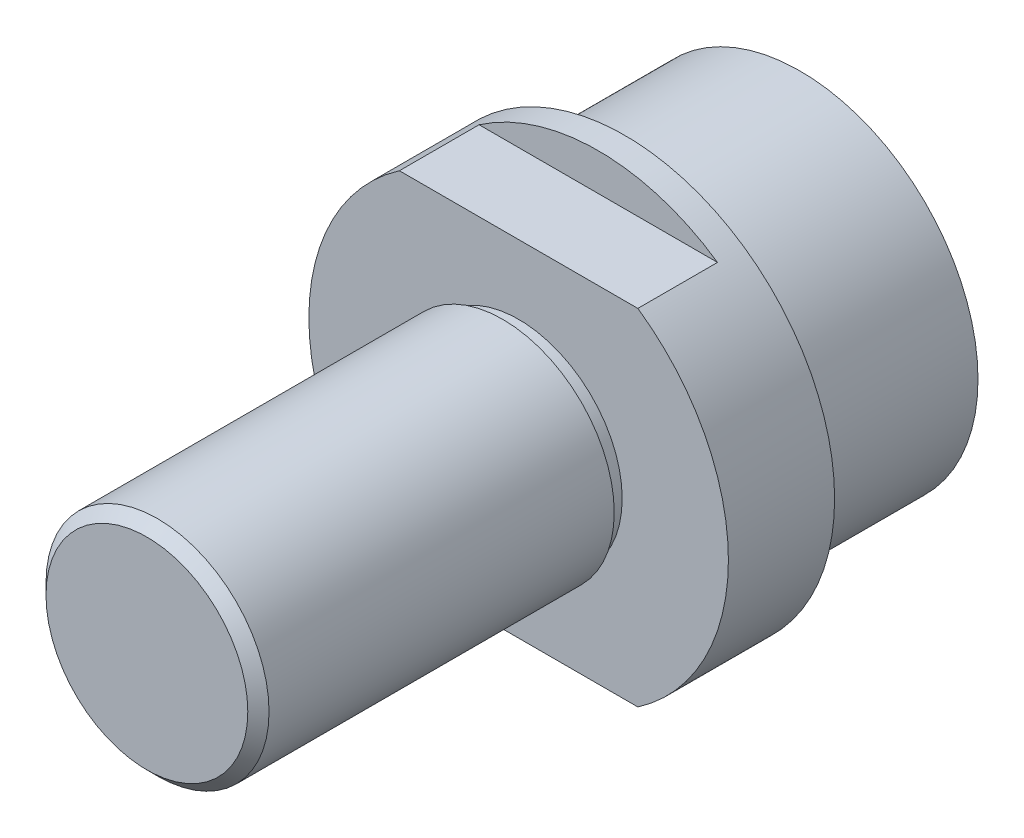
from build123d import *

# Parameters (mm, degrees)
SKETCH1_R           = 33.5
BOSS_EXTRUDE1_DEPTH = 33
SKETCH2_R           = 39.5
BOSS_EXTRUDE2_DEPTH = 20
CUT_EXTRUDE1_START  = -15
CUT_EXTRUDE1_DEPTH  = 15
SKETCH4_R           = 19.5
BOSS_EXTRUDE3_DEPTH = 3
SKETCH5_R           = 21
BOSS_EXTRUDE4_DEPTH = 67
CHAMFER1_SIZE       = 2


with BuildPart() as part:
    # Sketch1 → Boss-Extrude1 (new body)
    with BuildSketch(Plane.XY):
        Circle(SKETCH1_R)
    extrude(amount=BOSS_EXTRUDE1_DEPTH)

    # Sketch2 → Boss-Extrude2 (add)
    with BuildSketch(Plane.XY.offset(33)):
        Circle(SKETCH2_R)
    extrude(amount=BOSS_EXTRUDE2_DEPTH)

    # Sketch3 → Cut-Extrude1 (cut)
    with BuildSketch(Plane.XY.offset(53).offset(CUT_EXTRUDE1_START)):
        with BuildLine():
            Line((-22.449944321, 32.5), (22.449944321, 32.5))
            ThreePointArc((22.449944321, 32.5), (0, 39.5), (-22.449944321, 32.5))
        make_face()
        with BuildLine():
            Line((-22.449944321, -32.5), (22.449944321, -32.5))
            ThreePointArc((22.449944321, -32.5), (0, -39.5), (-22.449944321, -32.5))
        make_face()
    extrude(amount=CUT_EXTRUDE1_DEPTH, mode=Mode.SUBTRACT)

    # Sketch4 → Boss-Extrude3 (add)
    with BuildSketch(Plane.XY.offset(53)):
        Circle(SKETCH4_R)
    extrude(amount=BOSS_EXTRUDE3_DEPTH)

    # Sketch5 → Boss-Extrude4 (add)
    with BuildSketch(Plane.XY.offset(56)):
        Circle(SKETCH5_R)
    extrude(amount=BOSS_EXTRUDE4_DEPTH)

    # Chamfer1
    chamfer1_edges = [part.edges().sort_by_distance(p)[0] for p in [
        (-21, 0, 123),
    ]]
    chamfer(chamfer1_edges, length=CHAMFER1_SIZE)


solid = part.part
